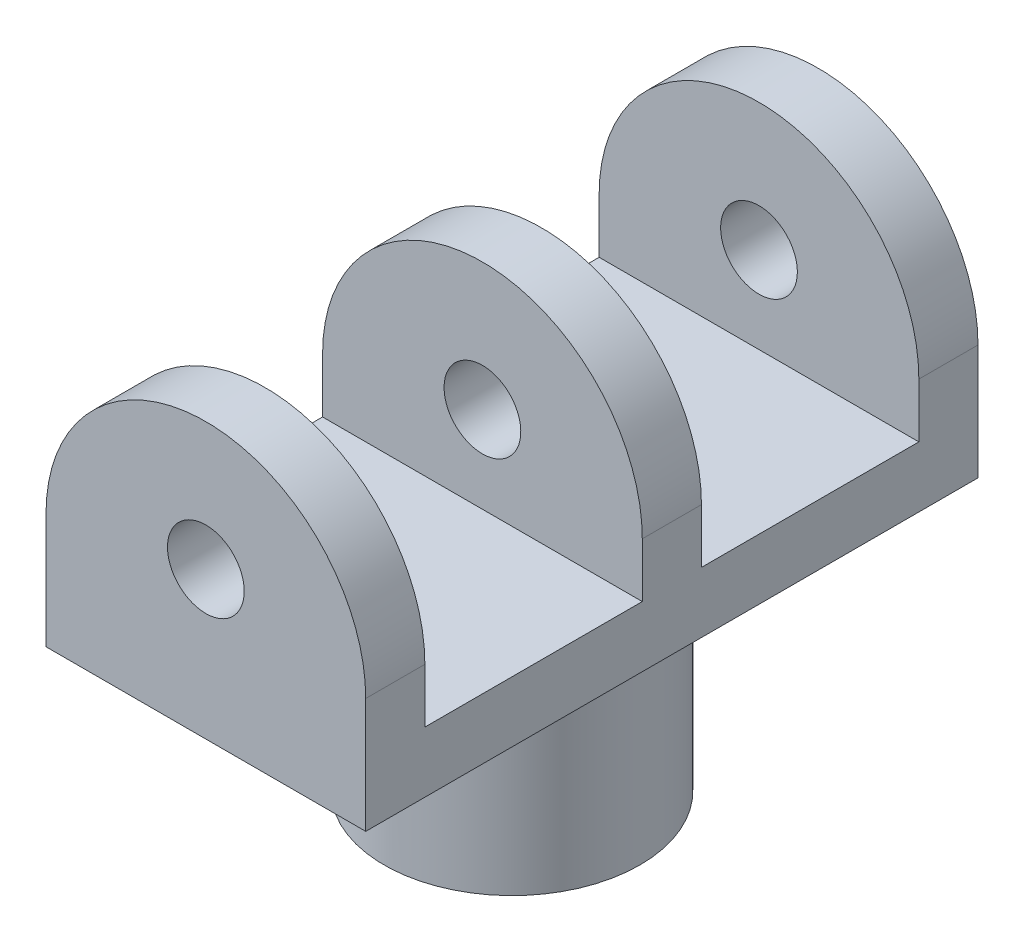
SolidWorks part; units mm, degrees
material "Q235"
ref_plane "Front Plane" through (0, 0, 0) normal (0, 0, 1) x (1, 0, 0)
ref_plane "Top Plane" through (0, 0, 0) normal (0, 1, 0) x (1, 0, 0)
ref_plane "Right Plane" through (0, 0, 0) normal (1, 0, 0) x (0, 0, -1)
sketch "Sketch1" plane through (0, 0, 0) normal (0, 0, 1) x (1, 0, 0)
  line L0 (0, 0) -> (0, 36)
  line L1 (100, 36) -> (100, 0)
  line L2 (100, 0) -> (0, 0)
  line L3 (50, 0) -> (50, 86.3359) construction
  arc A0 (0, 36) -> (100, 36) centre (50, 36) cw
  circle A2 centre (50, 46) radius 12
  dimension "D1" = 10
  dimension "D2" = 50
  dimension "D3" = 36
  dimension "D4" = 24
extrude "Boss-Extrude1" add sketch "Sketch1" along normal blind 191.5
sketch "Sketch2" plane through (0, 0, 0) normal (0, -1, 0) x (-1, 0, 0)
  line L0 (0, -191.5) -> (0, 0) construction
  line L1 (0, 0) -> (-100, 0) construction
  circle A0 centre (-50, -95.75) radius 40
  dimension "D1" = 80
  dimension "D2" = 50
  dimension "D3" = 95.75
extrude "Boss-Extrude2" add sketch "Sketch2" along normal blind 62
cosmetic thread "Cosmetic Thread1" parameters "D2"=79
sketch "Sketch3" plane through (0, 0, 0) normal (1, 0, 0) x (0, 0, -1)
  line L0 (-18.5, 86) -> (-18.5, 19)
  line L1 (0, 86) -> (-191.5, 86) construction
  line L2 (-18.5, 19) -> (-86.5, 19)
  line L3 (-86.5, 19) -> (-86.5, 86)
  line L4 (-86.5, 86) -> (-18.5, 86)
  line L5 (-105, 86) -> (-105, 19)
  line L6 (-105, 19) -> (-173, 19)
  line L7 (-173, 19) -> (-173, 86)
  line L8 (-173, 86) -> (-105, 86)
  line L9 (-191.5, 86) -> (-191.5, 36) construction
  dimension "D1" = 68
  dimension "D2" = 18.5
  dimension "D3" = 18.5
  dimension "D4" = 68
  dimension "D5" = 67
  dimension "D6" = 67
extrude "Cut-Extrude5" cut sketch "Sketch3" along normal through all
sketch "Sketch4" plane through (0, 0, 0) normal (0, 0, 1) x (1, 0, 0)
  line L0 (10, -62) -> (90, -62) construction
  line L1 (50, -62) -> (50, -6.8034) construction
  circle A0 centre (50, -32) radius 11
  dimension "D1" = 22
  dimension "D2" = 30
extrude "Cut-Extrude8" cut sketch "Sketch4" against normal through all and the other way through all
